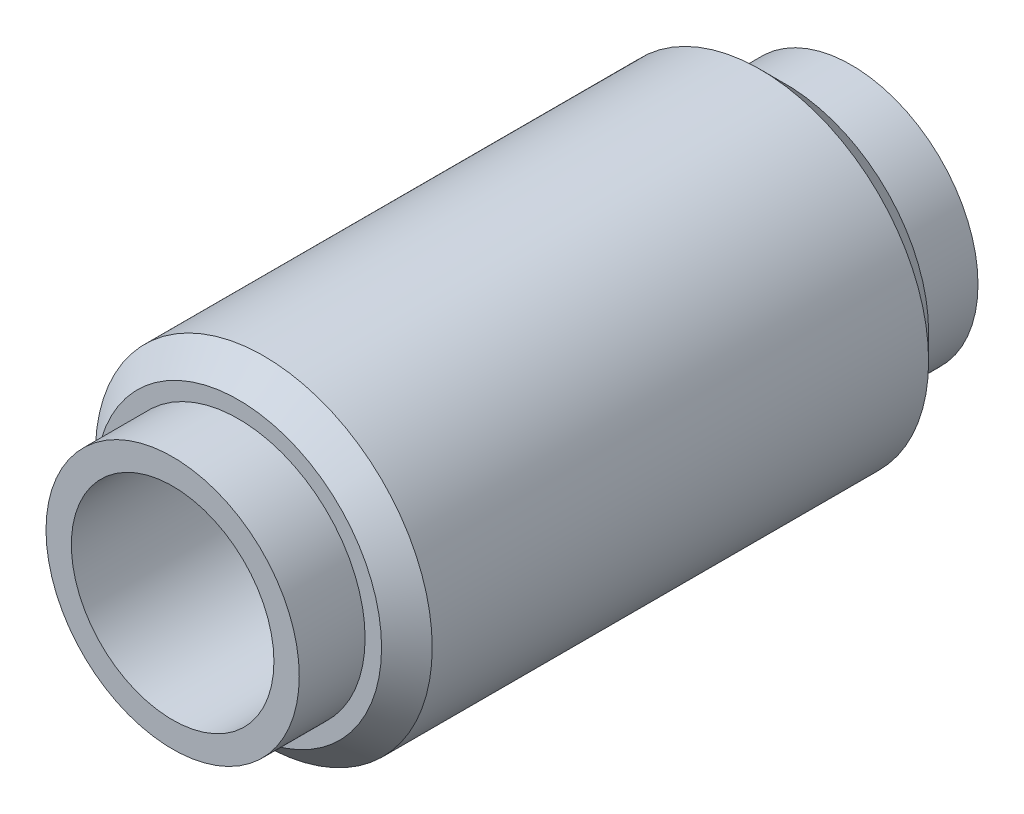
SolidWorks part; units mm, degrees
ref_plane "Front Plane" through (0, 0, 0) normal (0, 0, 1) x (1, 0, 0)
ref_plane "Top Plane" through (0, 0, 0) normal (0, 1, 0) x (1, 0, 0)
ref_plane "Right Plane" through (0, 0, 0) normal (1, 0, 0) x (0, 0, -1)
sketch "Sketch1" plane through (0, 0, 0) normal (0, 0, 1) x (1, 0, 0)
  circle A0 centre (0, 0) radius 50
  dimension "D1" = 100
extrude "Boss-Extrude1" add sketch "Sketch1" along normal blind 26
sketch "Sketch2" plane through (0, 0, 26) normal (0, 0, 1) x (1, 0, 0)
  circle A0 centre (0, 0) radius 66.5
  dimension "D1" = 133
extrude "Boss-Extrude2" add sketch "Sketch2" along normal blind 216
sketch "Sketch3" plane through (0, 0, 242) normal (0, 0, 1) x (1, 0, 0)
  circle A0 centre (0, 0) radius 50
  dimension "D1" = 100
extrude "Boss-Extrude3" add sketch "Sketch3" along normal blind 26
sketch "Sketch4" plane through (0, 0, 268) normal (0, 0, 1) x (1, 0, 0)
  circle A0 centre (0, 0) radius 40
  dimension "D1" = 80
extrude "Cut-Extrude1" cut sketch "Sketch4" against normal blind 79
sketch "Sketch5" plane through (0, 0, 0) normal (0, 0, -1) x (-1, 0, 0)
  circle A0 centre (0, 0) radius 40
  dimension "D1" = 80
extrude "Cut-Extrude2" cut sketch "Sketch5" against normal blind 79
sketch "Sketch6" plane through (0, 0, 79) normal (0, 0, -1) x (-1, 0, 0)
  circle A0 centre (0, 0) radius 36.5
  dimension "D1" = 73
extrude "Cut-Extrude3" cut sketch "Sketch6" against normal through all
chamfer "Chamfer1" distance 10 angle 45 1 edges at (66.5, 0, 242)
chamfer "Chamfer2" distance 10 angle 45 1 edges at (66.5, 0, 26)
